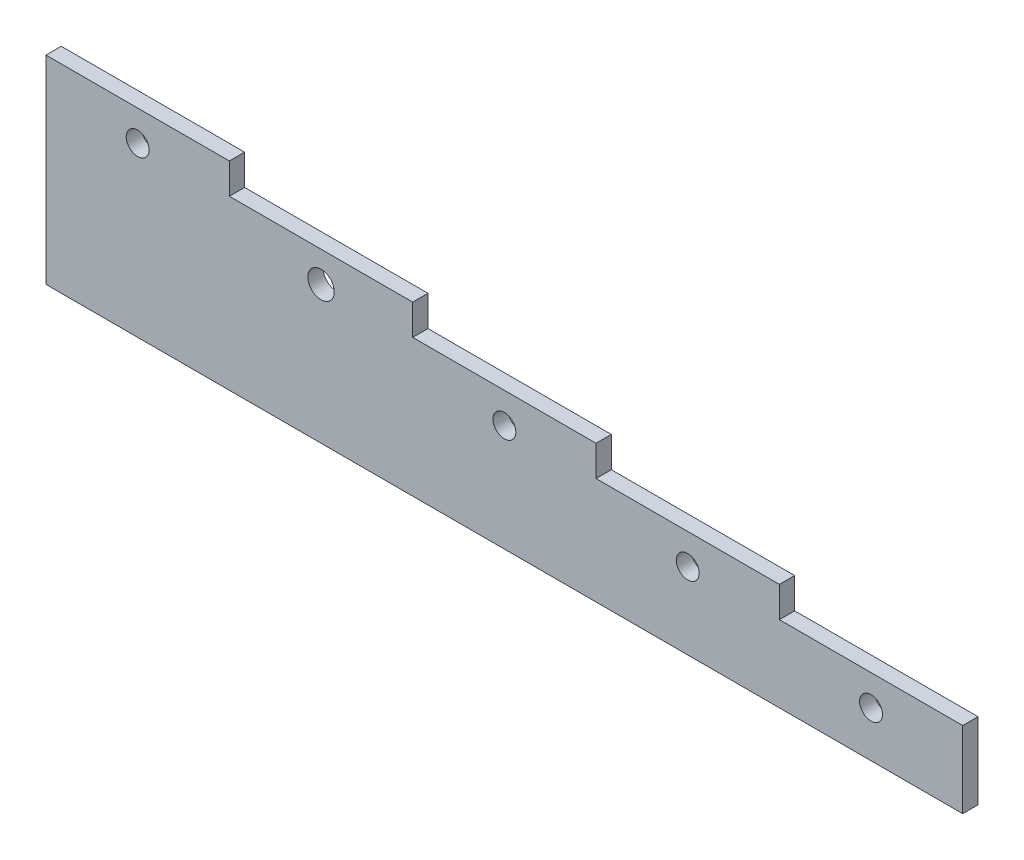
from build123d import *

# Parameters (mm, degrees)
SKETCH1_R           = 7.5
SKETCH1_R_2         = 8.652423936
BOSS_EXTRUDE1_DEPTH = 10


with BuildPart() as part:
    # Sketch1 → Boss-Extrude1 (new body)
    with BuildSketch(Plane.XY):
        Polygon((0, 0), (600, 0), (600, 50), (480, 50), (480, 70), (360, 70), (360, 90), (240, 90), (240, 110), (120, 110), (120, 130), (0, 130), align=None)
        with Locations((60, 110)):
            Circle(SKETCH1_R, mode=Mode.SUBTRACT)
        with Locations((180, 90)):
            Circle(SKETCH1_R_2, mode=Mode.SUBTRACT)
        with Locations((300, 70)):
            Circle(SKETCH1_R, mode=Mode.SUBTRACT)
        with Locations((420, 50)):
            Circle(SKETCH1_R, mode=Mode.SUBTRACT)
        with Locations((540, 30)):
            Circle(SKETCH1_R, mode=Mode.SUBTRACT)
    extrude(amount=BOSS_EXTRUDE1_DEPTH)


solid = part.part
